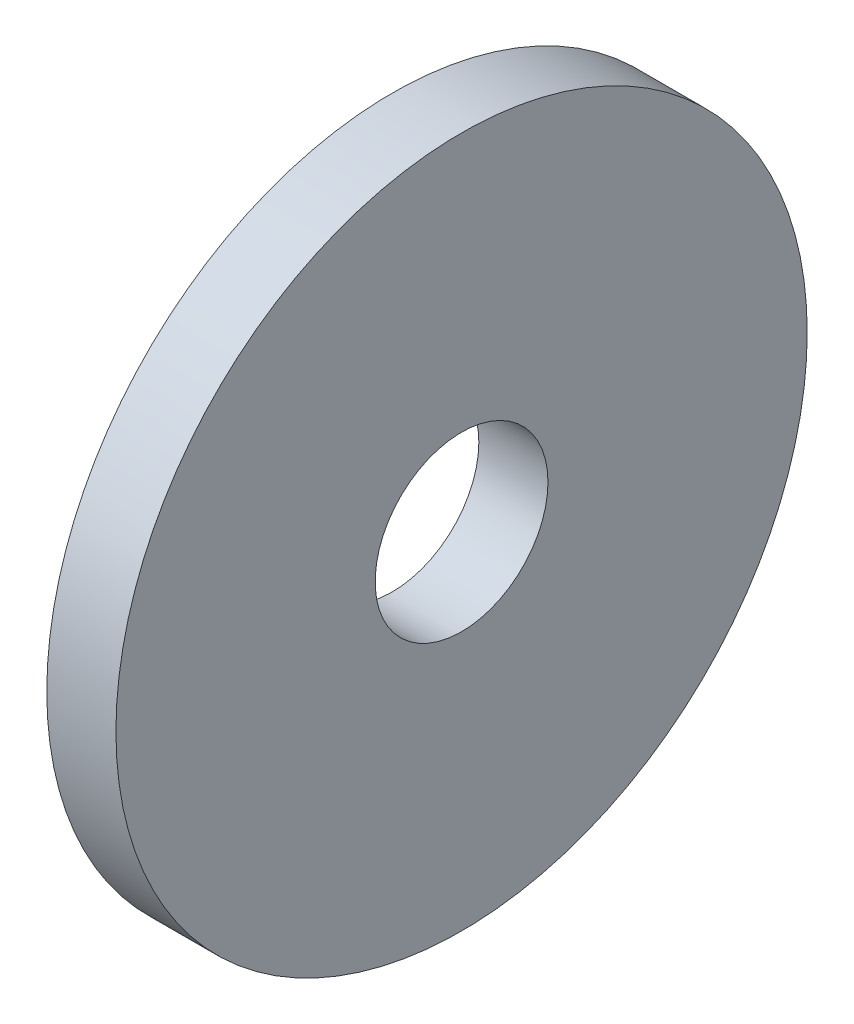
SolidWorks part; units mm, degrees
material "Q235B"
ref_plane "Front Plane" through (0, 0, 0) normal (0, 0, 1) x (1, 0, 0)
ref_plane "Top Plane" through (0, 0, 0) normal (0, 1, 0) x (1, 0, 0)
ref_plane "Right Plane" through (0, 0, 0) normal (1, 0, 0) x (0, 0, -1)
sketch "Sketch1" plane through (0, 0, 0) normal (1, 0, 0) x (0, 0, -1)
  circle A0 centre (0, 0) radius 5
  circle A1 centre (0, 0) radius 20
  dimension "D1" = 10
  dimension "D2" = 40
extrude "Boss-Extrude1" add sketch "Sketch1" along normal mid plane 4
